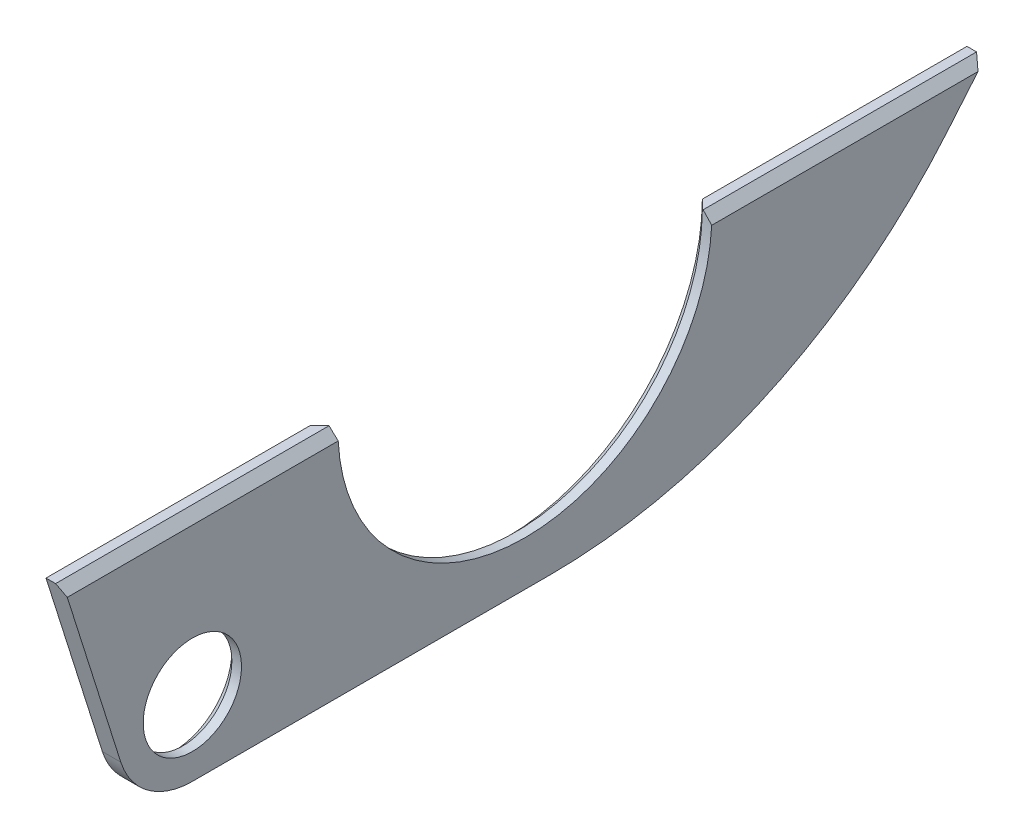
from build123d import *

# Parameters (mm, degrees)
BOSS_EXTRUDE1_DEPTH     = 12.5
CUT_EXTRUDE1_DEPTH      = 698.543905428
CUT_EXTRUDE1_DEPTH_BACK = 698.543905428
SKETCH2_R               = 66.5
FILLET1_R               = 700
CHAMFER1_SIZE           = 12
CHAMFER2_SIZE           = 12


with BuildPart() as part:
    # Sketch1 → Boss-Extrude1 (new, symmetric)
    with BuildSketch(Plane(origin=(0, 0, 0), x_dir=(0, 0, -1), z_dir=(1, 0, 0))):
        with BuildLine():
            Line((623, -1.2), (252.997154134, -1.2))
            ThreePointArc((252.997154134, -1.2), (0, -253), (-252.997154134, -1.2))
            Line((-252.997154134, -1.2), (-623, -1.2))
            Line((-623, -1.2), (-546.789689993, -242.561510288))
            ThreePointArc((-546.789689993, -242.561510288), (-510.001069598, -293.866486715), (-450, -313.5))
            Line((-450, -313.5), (360.949185183, -313.5))
            Line((360.949185183, -313.5), (623, -1.2))
        make_face()
    extrude(amount=BOSS_EXTRUDE1_DEPTH, both=True)

    # Sketch2 → Cut-Extrude1 (cut, two sides: drawn at the far end of the back side and taken through both)
    with BuildSketch(Plane(origin=(0, 0, 0), x_dir=(0, 0, -1), z_dir=(1, 0, 0)).offset(-CUT_EXTRUDE1_DEPTH_BACK)):
        with Locations((-450, -212)):
            Circle(SKETCH2_R)
    extrude(amount=CUT_EXTRUDE1_DEPTH + CUT_EXTRUDE1_DEPTH_BACK, mode=Mode.SUBTRACT)

    # Fillet1
    fillet1_edges = [part.edges().sort_by_distance(p)[0] for p in [
        (0, -313.5, -360.949185183),
    ]]
    fillet(fillet1_edges, radius=FILLET1_R)

    # Chamfer1
    chamfer1_edges = [part.edges().sort_by_distance(p)[0] for p in [
        (-12.5, -212, 516.5),
        (-12.5, -253, 0),
    ]]
    chamfer(chamfer1_edges, length=CHAMFER1_SIZE)

    # Chamfer2
    chamfer2_edges = [part.edges().sort_by_distance(p)[0] for p in [
        (12.5, -1.2, -437.998577067),
        (12.5, -1.2, 437.998577067),
    ]]
    chamfer(chamfer2_edges, length=CHAMFER2_SIZE)


solid = part.part
